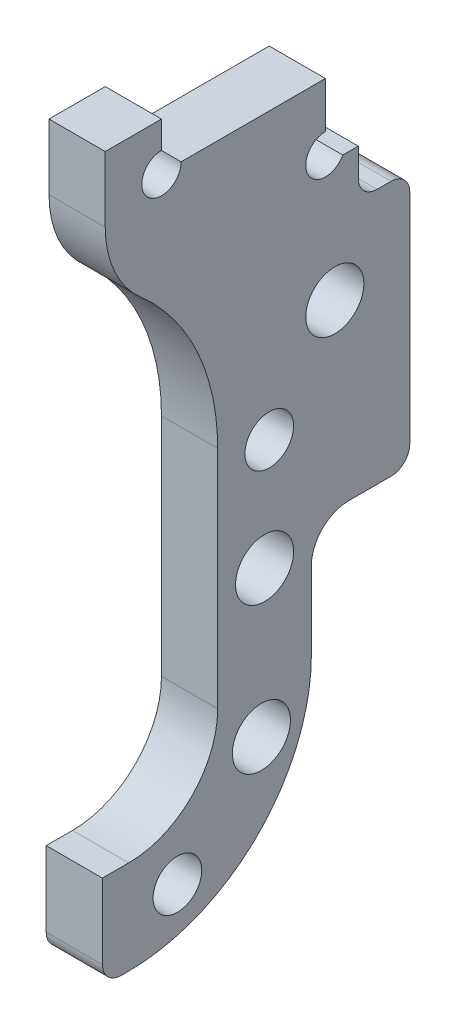
SolidWorks part; units mm, degrees
material "Thornel Mat VMA"
ref_plane "前视基准面" through (0, 0, 0) normal (0, 0, 1) x (1, 0, 0)
ref_plane "上视基准面" through (0, 0, 0) normal (0, 1, 0) x (1, 0, 0)
ref_plane "右视基准面" through (0, 0, 0) normal (1, 0, 0) x (0, 0, -1)
sketch "草图1" plane through (0, 0, 0) normal (1, 0, 0) x (0, 0, -1)
  line L0 (0, 0) -> (0, 48.25) construction
  line L1 (-9.25, 0) -> (-9.25, 19.75)
  line L2 (9.25, 0) -> (9.25, 19.75)
  line L3 (-24, -33.25) -> (-24, -37.75)
  line L4 (9.25, 19.75) -> (19.25, 19.75)
  line L5 (19.25, 19.75) -> (19.25, 0)
  line L6 (-24, -37.75) -> (6.7494, -37.75)
  line L7 (-24, -4.75) -> (-25.4, -4.75)
  line L8 (-25.4, -4.75) -> (-25.4, -14.75)
  line L9 (-25.4, -14.75) -> (-24, -14.75)
  line L10 (-19.25, 0) -> (-19.25, 19.75)
  line L11 (-19.25, 19.75) -> (-9.25, 19.75)
  line L12 (-24, 0) -> (11.1869, -2.1081) construction
  line L13 (-24, 0) -> (10.4888, -7.2859) construction
  line L14 (11.25, 3.1162) -> (11.25, 0) construction
  line L15 (-11.25, 0) -> (-11.25, 3.1162) construction
  line L16 (-24, 0) -> (-11.4381, -2.1822) construction
  line L17 (-24, 0) -> (-13.4117, -7.1029) construction
  line L18 (-24, -33.25) -> (-24, -14.75) construction
  line L19 (14, -37.75) -> (14, -27.25) construction
  line L20 (14, -27.25) -> (19.25, -27.25) construction
  line L21 (-24, 0) -> (-44, 0) construction
  line L22 (11.25, 3.1162) -> (11.1869, -2.1081) construction
  line L23 (10.4888, -7.2859) -> (11.1869, -2.1081) construction
  line L24 (-11.25, 3.1162) -> (-11.4381, -2.1822) construction
  line L25 (-11.4381, -2.1822) -> (-13.4117, -7.1029) construction
  line L26 (-25.4, -9.75) -> (-24, -9.75)
  line L27 (-14.25, 0) -> (-14.25, 19.75)
  line L28 (14.25, 0) -> (14.25, 19.75)
  line L29 (-17.8356, -34.7068) -> (-17.8356, -37.75) construction
  line L30 (-19.25, 19.75) -> (-19.25, 48.25)
  line L31 (-19.25, 48.25) -> (-9.25, 48.25)
  line L32 (19.25, 48.25) -> (19.25, 19.75)
  line L33 (9.25, 19.75) -> (9.25, 48.25)
  line L34 (-9.25, 19.75) -> (-9.25, 48.25)
  line L35 (9.25, 48.25) -> (19.25, 48.25)
  line L36 (-24, 0) -> (-1.8285, -34.25) construction
  line L37 (-24, 0) -> (16.5703, -4.3237) construction
  line L38 (-24, 0) -> (10.7567, -21.3684) construction
  line L39 (16.5703, -4.3237) -> (14.6157, -13.1708) construction
  line L40 (14.6157, -13.1708) -> (10.7567, -21.3684) construction
  line L41 (-14.25, 6.1162) -> (14.25, 6.1162)
  line L42 (5.2389, -39.7) -> (-24, -39.7)
  line L43 (-24, -39.7) -> (-24, -37.75)
  arc A0 (-24, -24) -> (0, 0) centre (-24, 0) ccw construction
  arc A1 (-24, -33.25) -> (9.25, 0) centre (-24, 0) ccw
  arc A2 (-24, -14.75) -> (-9.25, 0) centre (-24, 0) ccw
  arc A3 (5.2389, -39.7) -> (19.25, 0) centre (-44, 0) ccw
  arc A4 (-24, -4.75) -> (-19.25, 0) centre (-24, 0) ccw
  circle A5 centre (11.1869, -2.1081) radius 1.025
  circle A6 centre (10.4888, -7.2859) radius 1.025
  circle A7 centre (9.0331, -12.3036) radius 1.025
  circle A8 centre (6.8516, -17.0511) radius 1.025
  circle A9 centre (3.9925, -21.4239) radius 1.025
  circle A10 centre (0.5183, -25.3262) radius 1.025
  circle A11 centre (-3.4944, -28.672) radius 1.025
  circle A12 centre (-7.9577, -31.388) radius 1.025
  circle A13 centre (11.1869, -2.1081) radius 2.5 construction
  circle A14 centre (10.4888, -7.2859) radius 2.5 construction
  circle A15 centre (11.25, 3.1162) radius 1.025
  circle A16 centre (11.25, 3.1162) radius 2.5 construction
  arc A17 (11.25, 0) -> (-7.9577, -31.388) centre (-24, 0) cw construction
  arc A18 (-11.25, 0) -> (-22.1936, -12.6214) centre (-24, 0) cw construction
  circle A19 centre (-11.4381, -2.1822) radius 1.025
  circle A20 centre (-11.4381, -2.1822) radius 2.5 construction
  circle A21 centre (-13.4117, -7.1029) radius 1.025
  circle A22 centre (-17.2162, -10.7955) radius 1.025
  circle A23 centre (-22.1936, -12.6214) radius 1.025
  circle A25 centre (-11.25, 3.1162) radius 1.025
  circle A26 centre (-11.25, 3.1162) radius 2.5 construction
  circle A27 centre (-13.4117, -7.1029) radius 2.5 construction
  circle A28 centre (8, -29.75) radius 1.55
  circle A29 centre (9.0331, -12.3036) radius 2.5 construction
  circle A30 centre (6.8516, -17.0511) radius 2.5 construction
  circle A31 centre (3.9925, -21.4239) radius 2.5 construction
  circle A32 centre (0.5183, -25.3262) radius 2.5 construction
  circle A33 centre (-3.4944, -28.672) radius 2.5 construction
  circle A34 centre (-7.9577, -31.388) radius 2.5 construction
  circle A35 centre (-17.2162, -10.7955) radius 2.5 construction
  circle A36 centre (-22.1936, -12.6214) radius 2.5 construction
  arc A37 (-24, -9.75) -> (-14.25, 0) centre (-24, 0) ccw
  arc A38 (-24, -38.25) -> (14.25, 0) centre (-24, 0) ccw
  arc A39 (-24, -38.25) -> (14.25, 0) centre (-24, 0) ccw construction
  circle A40 centre (-12.7733, -33.4144) radius 1.025
  circle A41 centre (-17.8356, -34.7068) radius 1.025
  circle A42 centre (-12.7733, -33.4144) radius 2.5 construction
  circle A43 centre (-17.8356, -34.7068) radius 2.5 construction
  circle A44 centre (-21.4, -7.0349) radius 1.3
  circle A45 centre (-16.9174, -2.467) radius 1.55
  arc A48 (-16.9174, -2.467) -> (-21.4, -7.0349) centre (-24, 0) cw construction
  arc A49 (16.5703, -4.3237) -> (-1.8285, -34.25) centre (-24, 0) cw construction
  circle A50 centre (16.5703, -4.3237) radius 1.3
  circle A51 centre (14.6157, -13.1708) radius 1.55
  circle A52 centre (10.7567, -21.3684) radius 1.3
  circle A53 centre (-1.8285, -34.25) radius 1.3
  circle A55 centre (16.75, 5.25) radius 1.55
  circle A56 centre (-16.75, 5.25) radius 1.55
  circle A57 centre (-13, 15.75) radius 1.55
  circle A58 centre (-16.5, 11.05) radius 1.3
  circle A59 centre (16.5, 11.05) radius 1.3
  circle A60 centre (13, 15.75) radius 1.55
  dimension "D1" = 24
  dimension "D2" = 18.5
  dimension "D4" = 10
  dimension "D5" = 1.4
  dimension "D6" = 10
  dimension "D8" = 2.05
  dimension "D10" = 5
  dimension "D11" = 4
  dimension "D13" = 12.75
  dimension "D15" = 3.5
  dimension "D16" = 3.1
  dimension "D18" = 6
  dimension "D23" = 53
  dimension "D24" = 2.6
  dimension "D25" = 3.1
  dimension "D26" = 7.5
  dimension "D33" = 40.8
  dimension "D28" = 6.4
  dimension "D34" = 26
  dimension "D3" = 4.5
  dimension "D7" = 8.5
  dimension "D9" = 35.25
  dimension "D12" = 24
  dimension "D14" = 24.5
  dimension "D17" = 8
  dimension "D19" = 2.5
  dimension "D20" = 20
  dimension "D21" = 5
  dimension "D27" = 4
  dimension "D29" = 2.5
  dimension "D30" = 14.5
  dimension "D31" = 32
  dimension "D32" = 1.95
  dimension "D35" = 51
  dimension "D36" = 3
  dimension "D37" = 33
  dimension "D38" = 5.8
  dimension "D39" = 4
  dimension "D22" = 5
extrude "凸台-拉伸1" add sketch "草图1" along normal blind 3 contours L26 A37 L27 L11 L10 A4 L7 L8 A44 A45 A56 | L27 L41 L1 L11 | A38 L28
sketch "草图2" plane through (3, 0, 0) normal (1, 0, 0) x (0, 0, -1)
  line L0 (-19.25, 19.75) -> (-9.25, 19.75) construction
  line L1 (-9.25, 6.1162) -> (-9.25, 19.75) construction
  line L2 (-19.25, 19.75) -> (-11.75, 19.75)
  line L3 (-9.25, 6.1162) -> (-9.25, 19.75)
  line L4 (-9.25, 6.1162) -> (-9, 6.1162)
  line L5 (-9, 6.1162) -> (-9, 19.75)
  line L6 (-9, 19.75) -> (-9.25, 19.75)
  line L7 (-11.75, 19.75) -> (-11.75, 22.25)
  line L8 (-11.75, 22.25) -> (-12.5767, 22.25)
  line L9 (-13.5, 23.8) -> (-13.5, 26.25)
  line L13 (-25.25, 28.75) -> (-25.25, 25.25)
  line L14 (-13.5, 26.25) -> (-21.2, 26.25)
  line L15 (-22.25, 27.3) -> (-22.25, 28.75)
  line L16 (-22.25, 28.75) -> (-25.25, 28.75)
  line L17 (-19.25, 19.75) -> (-19.25, 12.0364)
  line L18 (-19.25, 0) -> (-19.25, 19.75) construction
  arc A1 (-13.5, 23.8) -> (-12.5767, 22.25) centre (-13.5, 22.75) ccw
  arc A2 (-22.25, 27.3) -> (-21.2, 26.25) centre (-22.25, 26.25) ccw
  arc A3 (-19.25, 12.0364) -> (-23.3526, 21.0713) centre (-31.25, 12.0364) ccw
  arc A4 (-25.25, 25.25) -> (-23.3526, 21.0713) centre (-19.7, 25.25) ccw
  point P22 (-17.1559, 24.3848)
  point P25 (-30.292, 32.8874)
  point P26 (-28.6046, 22.75)
  point P27 (-28.9796, 26.25)
  dimension "D1" = 1.05
  dimension "D6" = 12
  dimension "D12" = 5.55
  dimension "D2" = 13.5
  dimension "D3" = 0.25
  dimension "D4" = 2.5
  dimension "D5" = 1.75
  dimension "D7" = 6.5
  dimension "D8" = 2.5
  dimension "D9" = 0.5
  dimension "D10" = 3
  dimension "D11" = 3.5
  dimension "D13" = 6
extrude "凸台-拉伸2" add sketch "草图2" against normal through all
fillet "R2 圆角1" radius 2 1 edges at (1.5, 6.1162, 14.25)
fillet "R1 圆角1" radius 1 4 edges at (1.5, -9.75, 25.4) (1.5, 6.1162, 9) (1.5, 19.75, 11.75) (1.5, 19.75, 9)
